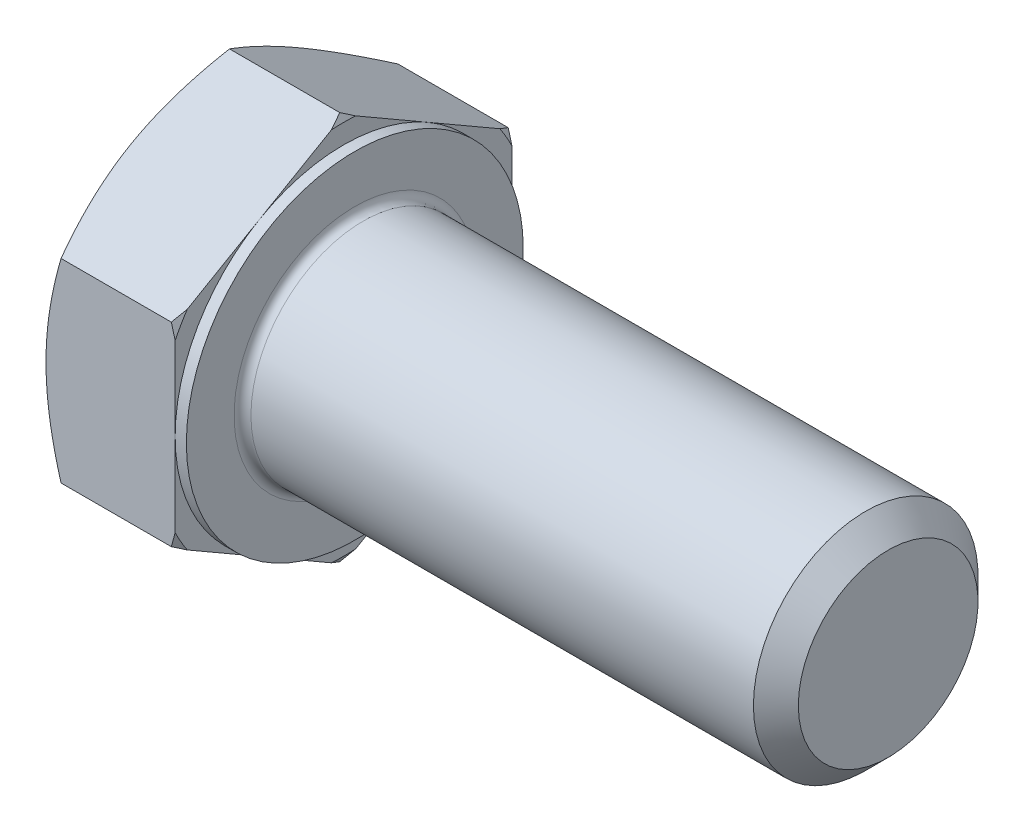
from build123d import *

# Parameters (mm, degrees)
BASE_EXTRUDE_DEPTH = 10
SKETCH4_W          = 0.8
SKETCH4_H          = 11.856406461
CHAMFER_2_SIZE     = 1.6
FILLET_2_R         = 0.6


with BuildPart() as part:
    # Sketch1 → Base-Extrude (new body)
    with BuildSketch(Plane(origin=(0, 0, 0), x_dir=(0, 0, -1), z_dir=(1, 0, 0))):
        Polygon((12, 6.92820323), (12, -6.92820323), (0, -13.856406461), (-12, -6.92820323), (-12, 6.92820323), (0, 13.856406461), align=None)
    extrude(amount=BASE_EXTRUDE_DEPTH)

    # Sketch2 → Boss-Revolve1 (revolve)
    with BuildSketch(Plane.XY, mode=Mode.PRIVATE) as boss_revolve1_sk:
        Polygon((0, 0), (48, 0), (48, 6.268), (48, 8), (27.8072, 8), (0, 8), align=None)
    revolve(boss_revolve1_sk.sketch.rotate(Axis((0, 0, 0), (1, 0, 0)), 90), axis=Axis((0, 0, 0), (1, 0, 0)))

    # Sketch3 → Cut-Revolve1 (revolve, cut)
    with BuildSketch(Plane.XY):
        Polygon((0, 12), (3.958548116, 18.856406461), (3.958548116, 23.856406461), (-10, 23.856406461), (-10, 12), align=None)
    revolve(axis=Axis((0, 0, 0), (1, 0, 0)), mode=Mode.SUBTRACT)

    # Sketch5 → Cut-Revolve2 (revolve, cut)
    with BuildSketch(Plane.XY):
        Polygon((10, 12), (6.041451884, 18.856406461), (6.041451884, 23.856406461), (16.041451884, 23.856406461), (16.041451884, 12), align=None)
    revolve(axis=Axis((0, 0, 0), (1, 0, 0)), mode=Mode.SUBTRACT)

    # Sketch4 → Cut-Revolve3 (revolve, cut)
    with BuildSketch(Plane.XY, mode=Mode.PRIVATE) as cut_revolve3_sk:
        with Locations((9.6, 17.928203231)):
            Rectangle(SKETCH4_W, SKETCH4_H)
    revolve(cut_revolve3_sk.sketch.rotate(Axis((0, 0, 0), (1, 0, 0)), 270), axis=Axis((0, 0, 0), (1, 0, 0)), mode=Mode.SUBTRACT)

    # Chamfer 2
    chamfer_2_edges = [part.edges().sort_by_distance(p)[0] for p in [
        (48, 0, -8),
    ]]
    chamfer(chamfer_2_edges, length=CHAMFER_2_SIZE)

    # Fillet 2
    fillet_2_edges = [part.edges().sort_by_distance(p)[0] for p in [
        (10, 0, -8),
    ]]
    fillet(fillet_2_edges, radius=FILLET_2_R)


solid = part.part
